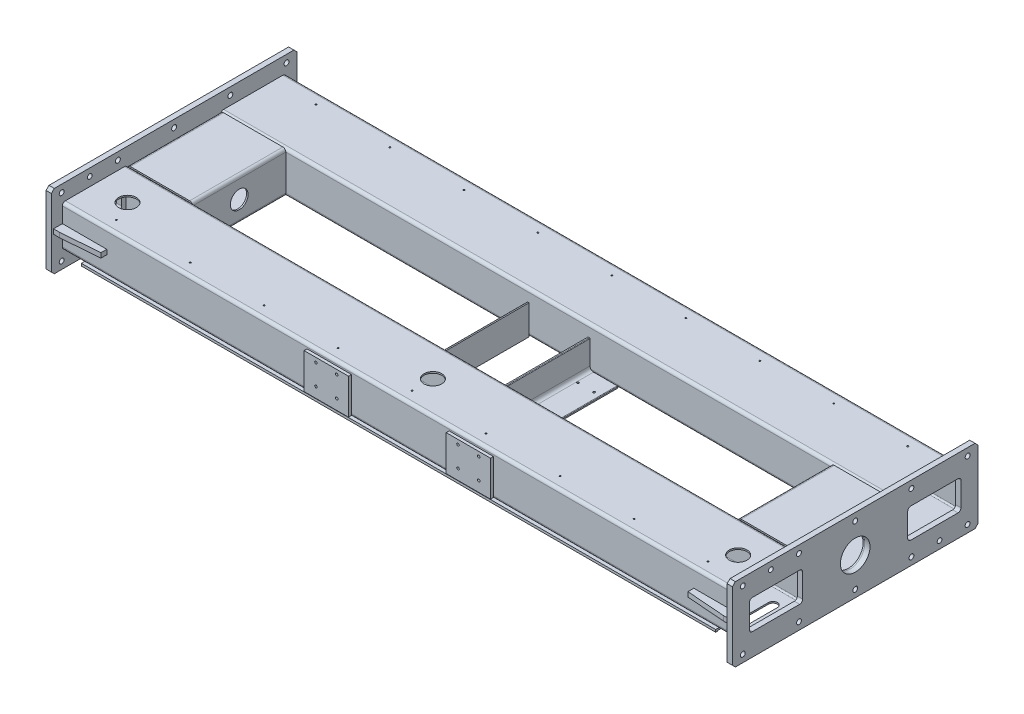
SolidWorks part; units mm, degrees
material "Q235A (2)"
ref_plane "前视基准面" through (0, 0, 0) normal (0, 0, 1) x (1, 0, 0)
ref_plane "上视基准面" through (0, 0, 0) normal (0, 1, 0) x (1, 0, 0)
ref_plane "右视基准面" through (0, 0, 0) normal (1, 0, 0) x (0, 0, -1)
sketch3d "3D草图1"
  line L0 (0, 0, 0) -> (2064, 0, 0)
  line L1 (0, 0, 0) -> (0, 0, -535)
  line L2 (2064, 0, 0) -> (2064, 0, -535)
  line L3 (0, 0, -535) -> (2064, 0, -535)
  line L4 (1032, 0, -535) -> (1032, 0, 0) construction
  line L5 (1132, 0, -535) -> (1132, 0, 0)
  line L6 (932, 0, -535) -> (932, 0, 0)
  line L15 (1132, 0, -535) -> (1132, 20, -535)
  line L16 (1132, 0, 0) -> (1132, 20, 0)
  line L17 (932, 0, 0) -> (932, 20, 0)
  line L18 (932, 0, -535) -> (932, 20, -535)
  line L19 (1132, 20, -535) -> (1132, 20, 0)
  line L20 (932, 20, 0) -> (932, 20, -535)
  line L21 (1132, 0, -535) -> (1132, -70, -535)
  line L22 (1132, 0, 0) -> (1132, -70, 0)
  line L23 (932, 0, 0) -> (932, -70, 0)
  line L24 (932, 0, -535) -> (932, -70, -535)
  line L25 (1132, -70, -535) -> (1132, -70, 0)
  line L26 (932, -70, 0) -> (932, -70, -535)
  dimension "D1" = 2064
  dimension "D2" = 535
  dimension "D3" = 200
  dimension "D4" = 100
  dimension "D5" = 20
  dimension "D6" = 70
other "矩型管 220×140×5(1)"
ref_plane "基准面1" through (0, 0, 0) normal (1, 0, 0) x (0, 1, 0)
sketch "Sketch11" plane through (0, 0, 0) normal (1, 0, 0) x (0, 1, 0)
  line L0 (-60, -105) -> (60, -105)
  line L1 (-65, -100) -> (-65, 100)
  line L2 (60, 105) -> (-60, 105)
  line L3 (65, 100) -> (65, -100)
  line L4 (-60, -110) -> (60, -110)
  line L5 (-70, -100) -> (-70, 100)
  line L6 (60, 110) -> (-60, 110)
  line L7 (70, 100) -> (70, -100)
  arc A0 (70, 100) -> (60, 110) centre (60, 100) ccw
  arc A1 (60, -110) -> (70, -100) centre (60, -100) ccw
  arc A2 (-70, -100) -> (-60, -110) centre (-60, -100) ccw
  arc A3 (-60, 110) -> (-70, 100) centre (-60, 100) ccw
  arc A4 (-60, 105) -> (-65, 100) centre (-60, 100) ccw
  arc A5 (65, 100) -> (60, 105) centre (60, 100) ccw
  arc A6 (60, -105) -> (65, -100) centre (60, -100) ccw
  arc A7 (-65, -100) -> (-60, -105) centre (-60, -100) ccw
  point P0 (0, 110)
  point P1 (70, 0)
  point P2 (0, -110)
  point P3 (-70, 0)
  point P4 (-70, 110)
  point P5 (70, 110)
  point P6 (70, -110)
  point P7 (-70, -110)
  point P8 (0, 0)
  point P33 (0, 0)
sketch "草图3" plane through (-110, 0, 0) normal (-1, 0, 0) x (0, 0, 1)
  line L0 (0, 0) -> (-535, 0) construction
  line L5 (-682.5, -125) -> (147.5, -125)
  line L6 (-682.5, -125) -> (-682.5, 125)
  line L11 (-682.5, 125) -> (147.5, 125)
  line L12 (147.5, -125) -> (147.5, 125)
  line L13 (-267.5, 125) -> (-267.5, -125) construction
  line L14 (-682.5, 0) -> (147.5, 0) construction
  point P0 (-267.5, 0)
  dimension "D1" = 250
  dimension "D2" = 830
extrude "凸台-拉伸1" add sketch "草图3" along normal blind 18 separate body
sketch "草图21" plane through (2174, 0, 0) normal (1, 0, 0) x (0, 0, -1)
  line L4 (-147.5, 125) -> (-147.5, -125)
  line L5 (-147.5, -125) -> (682.5, -125)
  line L6 (682.5, -125) -> (682.5, 125)
  line L7 (682.5, 125) -> (-147.5, 125)
  line L8 (-147.5, 125) -> (-147.5, -125)
  line L9 (-147.5, -125) -> (682.5, -125)
  line L10 (682.5, -125) -> (682.5, 125)
  line L11 (682.5, 125) -> (-147.5, 125)
  dimension "D1" = 0
extrude "凸台-拉伸4" add sketch "草图21" along normal blind 18 separate body
sketch "草图15" plane through (0, -70, 0) normal (0, -1, 0) x (1, 0, 0)
  line L0 (0, 0) -> (2064, 0) construction
  line L1 (-40, 91) -> (2104, 91) construction
  line L2 (-40, 116) -> (2104, 116)
  line L3 (-40, 116) -> (-40, 66)
  line L4 (-40, 66) -> (2104, 66)
  line L5 (2104, 116) -> (2104, 66)
  line L6 (-40, -91) -> (2104, -91) construction
  line L7 (2104, -116) -> (2104, -66)
  line L8 (-40, -66) -> (2104, -66)
  line L9 (-40, -116) -> (-40, -66)
  line L10 (-40, -116) -> (2104, -116)
  line L12 (1032, -110) -> (1032, 395.9711) construction
  line L13 (2174, -110) -> (-110, -110) construction
  line L14 (2104, -91) -> (-40, -91) construction
  line L24 (1032, -645) -> (1032, 538.6516) construction
  line L25 (2174, -645) -> (-110, -645) construction
  line L26 (-110, -425) -> (-110, -110) construction
  dimension "D1" = 70
  dimension "D2" = 50
  dimension "D3" = 182
extrude "凸台-拉伸3" add sketch "草图15" along normal blind 8 separate body
ref_plane "基准面3" through (0, 0, 80) normal (0, 0, 1) x (1, 0, 0)
ref_plane "基准面5" through (1032, 0, 0) normal (1, 0, 0) x (0, 0, -1)
sketch "草图22" plane through (0, -78, 0) normal (0, -1, 0) x (1, 0, 0)
  line L0 (-40, 116) -> (-40, 66) construction
  line L1 (-40, 66) -> (2104, 66)
  line L2 (-40, 66) -> (-40, 110)
  line L3 (-40, 110) -> (2104, 110)
  line L4 (2104, 66) -> (2104, 110)
  line L5 (-40, 66) -> (2104, 66) construction
  line L6 (2104, 66) -> (2104, 116) construction
  line L7 (2104, -66) -> (-40, -66) construction
  line L8 (-40, -66) -> (2104, -66)
  line L9 (-40, -66) -> (-40, -110)
  line L10 (-40, -110) -> (2104, -110)
  line L11 (2104, -66) -> (2104, -110)
  line L12 (2104, -116) -> (2104, -66) construction
  line L13 (0, 0) -> (2064, 0) construction
  dimension "D1" = 220
extrude "切除-拉伸1" cut sketch "草图22" against normal blind 2
hole_wizard "M8 螺纹孔1" positions "草图24" profile "草图25" tap size "M8" standard "GB"
sketch "草图24" plane through (0, -76, 0) normal (0, -1, 0) x (-1, 0, 0)
  line L0 (-2064, 0) -> (0, 0) construction
  line L2 (-2104, 91) -> (40, 91) construction
  line L3 (-2104, 110) -> (-2104, 66) construction
  line L4 (40, 66) -> (40, 110) construction
  line L6 (-2104, -91) -> (40, -91) construction
  line L7 (-1032, 91) -> (-1032, -91) construction
  point P21 (-26, 91)
  point P23 (-76, 91)
  point P25 (-176, 91)
  point P27 (-376, 91)
  point P29 (-576, 91)
  point P31 (-776, 91)
  point P34 (-876, 91)
  point P37 (-876, -91)
  point P38 (-776, -91)
  point P39 (-576, -91)
  point P40 (-376, -91)
  point P41 (-176, -91)
  point P42 (-76, -91)
  point P43 (-26, -91)
  point P44 (-2038, -91)
  point P45 (-1988, -91)
  point P46 (-1888, -91)
  point P47 (-1688, -91)
  point P48 (-1488, -91)
  point P49 (-1288, -91)
  point P50 (-1188, -91)
  point P51 (-1188, 91)
  point P52 (-1288, 91)
  point P53 (-1488, 91)
  point P54 (-1688, 91)
  point P55 (-1888, 91)
  point P56 (-1988, 91)
  point P57 (-2038, 91)
  dimension "D1" = 182
  dimension "D2" = 66
  dimension "D3" = 50
  dimension "D4" = 100
  dimension "D5" = 200
  dimension "D6" = 200
  dimension "D7" = 200
  dimension "D8" = 100
sketch "草图25" plane through (2038, -76, -91) normal (1, 0, 0) x (0, 0, -1)
  line L0 (0, 0) -> (0, 24.2929)
  line L1 (0, 24.2929) -> (3.4, 22.25)
  line L2 (3.4, 22.25) -> (3.4, 0)
  line L5 (3.4, 0) -> (0, 0)
  line L10 (0, 24.2929) -> (-3.4, 22.25) construction
  line L11 (0, -6.35) -> (0, 107.95) construction
  dimension "螺纹孔钻头直径" = 6.8
  dimension "螺纹孔钻头深度" = 22.25
  dimension "导头角度" = 118
cosmetic thread "孔螺蚊线1" parameters "D1"=11, "D2"=8
cosmetic thread "孔螺蚊线2" parameters "D1"=11, "D2"=8
cosmetic thread "孔螺蚊线3" parameters "D1"=11, "D2"=8
cosmetic thread "孔螺蚊线4" parameters "D1"=11, "D2"=8
cosmetic thread "孔螺蚊线5" parameters "D1"=11, "D2"=8
cosmetic thread "孔螺蚊线6" parameters "D1"=11, "D2"=8
cosmetic thread "孔螺蚊线7" parameters "D1"=11, "D2"=8
cosmetic thread "孔螺蚊线8" parameters "D1"=11, "D2"=8
cosmetic thread "孔螺蚊线9" parameters "D1"=11, "D2"=8
cosmetic thread "孔螺蚊线10" parameters "D1"=11, "D2"=8
cosmetic thread "孔螺蚊线11" parameters "D1"=11, "D2"=8
cosmetic thread "孔螺蚊线12" parameters "D1"=11, "D2"=8
cosmetic thread "孔螺蚊线13" parameters "D1"=11, "D2"=8
cosmetic thread "孔螺蚊线14" parameters "D1"=11, "D2"=8
cosmetic thread "孔螺蚊线15" parameters "D1"=11, "D2"=8
cosmetic thread "孔螺蚊线16" parameters "D1"=11, "D2"=8
cosmetic thread "孔螺蚊线17" parameters "D1"=11, "D2"=8
cosmetic thread "孔螺蚊线18" parameters "D1"=11, "D2"=8
cosmetic thread "孔螺蚊线19" parameters "D1"=11, "D2"=8
cosmetic thread "孔螺蚊线20" parameters "D1"=11, "D2"=8
cosmetic thread "孔螺蚊线21" parameters "D1"=11, "D2"=8
cosmetic thread "孔螺蚊线22" parameters "D1"=11, "D2"=8
cosmetic thread "孔螺蚊线23" parameters "D1"=11, "D2"=8
cosmetic thread "孔螺蚊线24" parameters "D1"=11, "D2"=8
cosmetic thread "孔螺蚊线25" parameters "D1"=11, "D2"=8
cosmetic thread "孔螺蚊线26" parameters "D1"=11, "D2"=8
cosmetic thread "孔螺蚊线27" parameters "D1"=11, "D2"=8
cosmetic thread "孔螺蚊线28" parameters "D1"=11, "D2"=8
sketch "草图27" plane through (2192, 0, 0) normal (1, 0, 0) x (0, 0, -1)
  line L0 (682.5, 0) -> (-147.5, 0) construction
  line L1 (682.5, -125) -> (682.5, 125) construction
  line L2 (-147.5, 125) -> (-147.5, -125) construction
  line L3 (535, 70) -> (535, -70) construction
  line L4 (635, 70) -> (435, 70) construction
  line L5 (435, -70) -> (635, -70) construction
  line L6 (0, 70) -> (0, -70) construction
  line L7 (100, 70) -> (-100, 70) construction
  line L8 (-100, -70) -> (100, -70) construction
  line L9 (267.5, 125) -> (267.5, -125) construction
  line L10 (455, 50) -> (615, 50)
  line L11 (445, 40) -> (445, -40)
  line L12 (455, -50) -> (615, -50)
  line L13 (625, 40) -> (625, -40)
  line L14 (535, -50) -> (535, 50) construction
  line L15 (445, 0) -> (625, 0) construction
  line L16 (682.5, 125) -> (-147.5, 125) construction
  line L17 (-147.5, -125) -> (682.5, -125) construction
  line L18 (90, 0) -> (-90, 0) construction
  line L19 (0, -50) -> (0, 50) construction
  line L20 (0, 70) -> (0, -70) construction
  line L21 (-90, 40) -> (-90, -40)
  line L22 (80, -50) -> (-80, -50)
  line L23 (90, 40) -> (90, -40)
  line L24 (80, 50) -> (-80, 50)
  arc A0 (-80, 50) -> (-90, 40) centre (-80, 40) ccw
  arc A1 (-90, -40) -> (-80, -50) centre (-80, -40) ccw
  arc A2 (80, -50) -> (90, -40) centre (80, -40) ccw
  arc A3 (80, 50) -> (90, 40) centre (80, 40) cw
  arc A4 (455, 50) -> (445, 40) centre (455, 40) ccw
  arc A5 (625, -40) -> (615, -50) centre (615, -40) cw
  arc A6 (455, -50) -> (445, -40) centre (455, -40) cw
  arc A7 (615, 50) -> (625, 40) centre (615, 40) cw
  point P18 (535, 0)
  point P36 (0, 0)
  point P39 (-90, 50)
  point P42 (-90, -50)
  point P45 (90, -50)
  point P48 (90, 50)
  point P51 (445, 50)
  point P54 (625, -50)
  point P57 (445, -50)
  point P60 (625, 50)
  dimension "D3" = 10
  dimension "D1" = 100
  dimension "D2" = 180
extrude "切除-拉伸2" cut sketch "草图27" against normal through all
sketch "草图28" plane through (-128, 0, 0) normal (-1, 0, 0) x (0, 0, 1)
  line L0 (-90, -40) -> (-90, 40) construction
  line L1 (-80, 50) -> (80, 50) construction
  line L2 (90, 40) -> (90, -40) construction
  line L3 (80, -50) -> (-80, -50) construction
  line L4 (-90, -40) -> (-90, 40)
  line L5 (-80, 50) -> (80, 50)
  line L6 (90, 40) -> (90, -40)
  line L7 (80, -50) -> (-80, -50)
  line L8 (-625, -40) -> (-625, 40) construction
  line L9 (-455, -50) -> (-615, -50) construction
  line L10 (-445, 40) -> (-445, -40) construction
  line L11 (-615, 50) -> (-455, 50) construction
  line L20 (-625, -40) -> (-625, 40)
  line L21 (-455, -50) -> (-615, -50)
  line L22 (-445, 40) -> (-445, -40)
  line L23 (-615, 50) -> (-455, 50)
  arc A0 (-80, 50) -> (-90, 40) centre (-80, 40) ccw construction
  arc A1 (90, 40) -> (80, 50) centre (80, 40) ccw construction
  arc A2 (80, -50) -> (90, -40) centre (80, -40) ccw construction
  arc A3 (-90, -40) -> (-80, -50) centre (-80, -40) ccw construction
  arc A4 (-80, 50) -> (-90, 40) centre (-80, 40) ccw
  arc A5 (90, 40) -> (80, 50) centre (80, 40) ccw
  arc A6 (80, -50) -> (90, -40) centre (80, -40) ccw
  arc A7 (-90, -40) -> (-80, -50) centre (-80, -40) ccw
  arc A8 (-615, 50) -> (-625, 40) centre (-615, 40) ccw construction
  arc A9 (-625, -40) -> (-615, -50) centre (-615, -40) ccw construction
  arc A10 (-455, -50) -> (-445, -40) centre (-455, -40) ccw construction
  arc A11 (-445, 40) -> (-455, 50) centre (-455, 40) ccw construction
  arc A12 (-615, 50) -> (-625, 40) centre (-615, 40) ccw
  arc A13 (-625, -40) -> (-615, -50) centre (-615, -40) ccw
  arc A14 (-455, -50) -> (-445, -40) centre (-455, -40) ccw
  arc A15 (-445, 40) -> (-455, 50) centre (-455, 40) ccw
extrude "切除-拉伸3" cut sketch "草图28" against normal blind 25
sketch "草图29" plane through (0, -70, 0) normal (0, -1, 0) x (1, 0, 0)
  line L0 (0, 0) -> (2064, 0) construction
  line L1 (1107, 0) -> (957, 0) construction
  line L2 (1107, -45) -> (957, -45)
  line L3 (1107, 45) -> (957, 45)
  arc A0 (1107, -45) -> (1107, 45) centre (1107, 0) ccw
  arc A1 (957, 45) -> (957, -45) centre (957, 0) ccw
  point P6 (1032, 0)
  dimension "D1" = 90
  dimension "D2" = 150
extrude "切除-拉伸4" cut sketch "草图29" against normal blind 6
sketch "草图30" plane through (0, 0, 0) normal (0, 1, 0) x (1, 0, 0)
  line L8 (-128, 267.5) -> (2192, 267.5) construction
  line L9 (-128, -147.5) -> (-128, 682.5) construction
  line L10 (2192, 682.5) -> (2192, -147.5) construction
  line L17 (1032, 535) -> (1032, -585.4821) construction
  line L18 (0, 535) -> (2064, 535) construction
  line L19 (1032, -137.5) -> (1032, 137.5) construction
hole_wizard "Ø16.5 (16.5) 直径孔1" positions "草图32" profile "草图33" hole size "Ø16.5" standard "GB"
sketch "草图32" plane through (2192, 0, 0) normal (1, 0, 0) x (0, 0, -1)
  line L1 (647.5, -100) -> (-112.5, -100) construction
  line L2 (647.5, -100) -> (647.5, 100) construction
  line L3 (647.5, 100) -> (-112.5, 100) construction
  line L4 (-112.5, -100) -> (-112.5, 100) construction
  line L5 (267.5, 100) -> (267.5, -100) construction
  line L6 (647.5, 0) -> (-112.5, 0) construction
  line L8 (267.5, 125) -> (267.5, -125) construction
  line L9 (682.5, 125) -> (-147.5, 125) construction
  line L10 (-147.5, -125) -> (682.5, -125) construction
  line L11 (77.5, 100) -> (77.5, -100) construction
  line L13 (457.5, 100) -> (457.5, -100) construction
  point P2 (-112.5, 100)
  point P279 (647.5, -100)
  point P280 (647.5, 100)
  point P281 (-112.5, -100)
  point P283 (267.5, -100)
  point P285 (267.5, 100)
  point P308 (457.5, 100)
  point P310 (77.5, 100)
  point P314 (77.5, -100)
  point P317 (457.5, -100)
  point P319 (350.269, 181.4428)
  point P321 (350.269, 181.4428)
  dimension "D1" = 760
  dimension "D2" = 200
  dimension "D3" = 380
sketch "草图33" plane through (2192, 100, 112.5) normal (0, 1, 0) x (0, 0, -1)
  line L0 (0, 0) -> (0, 2320)
  line L1 (0, 2320) -> (8.25, 2320)
  line L2 (8.25, 2320) -> (8.25, 0)
  line L5 (8.25, 0) -> (0, 0)
  line L11 (0, -6.35) -> (0, 107.95) construction
  dimension "通孔孔直径" = 16.5
  dimension "通孔孔深度" = 2320
hole_wizard "大小mm 暗销孔1" positions "草图34" profile "草图35" hole size "Ø16.0" standard "GB" end condition through all
sketch "草图34" plane through (2192, 0, 0) normal (1, 0, 0) x (0, 0, -1)
  line L0 (-112.5, 100) -> (77.5, 100) construction
  line L2 (457.5, -100) -> (647.5, -100) construction
  point P13 (-17.5, 100)
  point P15 (552.5, -100)
sketch "草图35" plane through (2192, -100, -552.5) normal (0, 1, 0) x (0, 0, -1)
  line L0 (0, 0) -> (0, 2320)
  line L1 (0, 2320) -> (8, 2320)
  line L2 (8, 2320) -> (8, 0)
  line L5 (8, 0) -> (0, 0)
  line L11 (0, -6.35) -> (0, 107.95) construction
  dimension "通孔孔直径" = 16
  dimension "通孔孔深度" = 2320
chamfer "倒角1" distance 10 angle 45 4 edges at (2183, 125, -682.5) (2183, -125, -682.5) (2183, 125, 147.5) (2183, -125, 147.5)
chamfer "倒角2" distance 10 angle 45 4 edges at (-119, -125, 147.5) (-119, 125, 147.5) (-119, 125, -682.5) (-119, -125, -682.5)
ref_plane "基准面6" through (0, 0, -535) normal (0, 0, -1) x (-1, 0, 0)
other "等边角钢 10×6(4)"
ref_plane "基准面7" through (1132, -70, -535) normal (0, 0, 1) x (0, 1, 0)
sketch "Sketch1" plane through (1132, -70, -535) normal (0, 0, 1) x (0, 1, 0)
  line L0 (100, 0) -> (0, 0)
  line L1 (0, 0) -> (0, -100)
  line L2 (98, -6) -> (18, -6)
  line L3 (6, -18) -> (6, -98)
  line L4 (100, 0) -> (100, -4)
  line L5 (0, -100) -> (4, -100)
  arc A0 (100, -4) -> (98, -6) centre (98, -4) cw
  arc A1 (4, -100) -> (6, -98) centre (4, -98) ccw
  arc A2 (18, -6) -> (6, -18) centre (18, -18) ccw
  point P2 (50, 0)
  point P13 (0, -50)
  point P15 (0, 0)
  dimension "r1" = 2
  dimension "r" = 12
  dimension "b" = 100
  dimension "d" = 6
other "等边角钢 10×6(1)"
ref_plane "基准面8" through (932, -70, 0) normal (0, 0, 1) x (-1, 0, 0)
sketch "Sketch15" plane through (932, -70, 0) normal (0, 0, 1) x (-1, 0, 0)
  line L0 (100, 0) -> (0, 0)
  line L1 (0, 0) -> (0, -100)
  line L2 (98, -6) -> (18, -6)
  line L3 (6, -18) -> (6, -98)
  line L4 (100, 0) -> (100, -4)
  line L5 (0, -100) -> (4, -100)
  arc A0 (100, -4) -> (98, -6) centre (98, -4) cw
  arc A1 (4, -100) -> (6, -98) centre (4, -98) ccw
  arc A2 (18, -6) -> (6, -18) centre (18, -18) ccw
  point P2 (50, 0)
  point P13 (0, -50)
  point P15 (0, 0)
  dimension "r1" = 2
  dimension "r" = 12
  dimension "b" = 100
  dimension "d" = 6
other "剪裁/延伸1"
sketch "草图41" plane through (0, 0, 0) normal (0, 1, 0) x (1, 0, 0)
  line L0 (2174, -110) -> (-110, -110) construction
  line L1 (40, -110) -> (-110, -110)
  line L2 (-110, -110) -> (-110, -140)
  line L3 (-90, 675) -> (-110, 675)
  line L4 (40, -110) -> (40, -130)
  line L5 (40, -130) -> (-90, -140)
  line L6 (-90, -140) -> (-110, -140)
  line L7 (-110, -137.5) -> (-110, -147.5) construction
  line L8 (2174, -100) -> (-110, -100) construction
  line L9 (1032, 535) -> (1032, -585.4821) construction
  line L10 (-128, 267.5) -> (2192, 267.5) construction
  line L26 (40, 665) -> (-90, 675)
  line L27 (40, 645) -> (40, 665)
  line L28 (-110, 645) -> (-110, 675)
  line L29 (40, 645) -> (-110, 645)
  line L30 (2024, 645) -> (2174, 645)
  line L31 (2174, 645) -> (2174, 675)
  line L32 (2024, 645) -> (2024, 665)
  line L33 (2024, 665) -> (2154, 675)
  line L34 (2154, -140) -> (2174, -140)
  line L35 (2024, -130) -> (2154, -140)
  line L36 (2024, -110) -> (2024, -130)
  line L37 (2154, 675) -> (2174, 675)
  line L39 (2024, -110) -> (2174, -110)
  line L40 (2174, -140) -> (2174, -110)
  dimension "D1" = 20
  dimension "D2" = 150
  dimension "D3" = 20
  dimension "D4" = 40
extrude "凸台-拉伸7" add sketch "草图41" along normal mid plane 16 separate body
sketch "草图42" plane through (0, 70, 0) normal (0, 1, 0) x (1, 0, 0)
  line L0 (1032, 535) -> (1032, -585.4821) construction
  line L1 (32, -70) -> (2032, -70) construction
  line L2 (2174, -110) -> (2024, -110) construction
  point P6 (782, -70)
  point P9 (1032, -70)
  point P10 (532, -70)
  point P11 (1782, -70)
  point P13 (32, -70)
  point P14 (1532, -70)
  point P15 (282, -70)
  point P16 (1282, -70)
  dimension "D1" = 40
  dimension "D2" = 250
  dimension "D3" = 250
  dimension "D4" = 250
  dimension "D5" = 250
hole_wizard "M6 螺纹孔2" positions "草图47" profile "草图48" tap size "M6" standard "GB"
sketch "草图47" plane through (0, 70, 0) normal (0, 1, 0) x (1, 0, 0)
  line L1 (1032, 535) -> (1032, -70) construction
  line L2 (-128, 267.5) -> (2192, 267.5) construction
  line L3 (32, 605) -> (2032, 605) construction
  point P5 (1032, -70)
  point P13 (32, -70)
  point P16 (282, -70)
  point P19 (532, -70)
  point P22 (782, -70)
  point P27 (1282, -70)
  point P30 (1532, -70)
  point P33 (1782, -70)
  point P36 (2032, -70)
  point P40 (2032, 605)
  point P41 (1782, 605)
  point P42 (1532, 605)
  point P43 (1282, 605)
  point P44 (782, 605)
  point P45 (532, 605)
  point P46 (282, 605)
  point P47 (32, 605)
  point P48 (1032, 605)
sketch "草图48" plane through (1032, 70, -605) normal (1, 0, 0) x (0, 0, 1)
  line L0 (0, 0) -> (0, 18.5022)
  line L1 (0, 18.5022) -> (2.5, 17)
  line L2 (2.5, 17) -> (2.5, 0)
  line L5 (2.5, 0) -> (0, 0)
  line L10 (0, 18.5022) -> (-2.5, 17) construction
  line L11 (0, -6.35) -> (0, 107.95) construction
  dimension "螺纹孔钻头直径" = 5
  dimension "螺纹孔钻头深度" = 17
  dimension "导头角度" = 118
cosmetic thread "孔螺蚊线45" parameters "D1"=5, "D2"=6
cosmetic thread "孔螺蚊线46" parameters "D1"=5, "D2"=6
cosmetic thread "孔螺蚊线47" parameters "D1"=5, "D2"=6
cosmetic thread "孔螺蚊线48" parameters "D1"=5, "D2"=6
cosmetic thread "孔螺蚊线49" parameters "D1"=5, "D2"=6
cosmetic thread "孔螺蚊线50" parameters "D1"=5, "D2"=6
cosmetic thread "孔螺蚊线51" parameters "D1"=5, "D2"=6
cosmetic thread "孔螺蚊线52" parameters "D1"=5, "D2"=6
cosmetic thread "孔螺蚊线53" parameters "D1"=5, "D2"=6
cosmetic thread "孔螺蚊线54" parameters "D1"=5, "D2"=6
cosmetic thread "孔螺蚊线55" parameters "D1"=5, "D2"=6
cosmetic thread "孔螺蚊线56" parameters "D1"=5, "D2"=6
cosmetic thread "孔螺蚊线57" parameters "D1"=5, "D2"=6
cosmetic thread "孔螺蚊线58" parameters "D1"=5, "D2"=6
cosmetic thread "孔螺蚊线59" parameters "D1"=5, "D2"=6
cosmetic thread "孔螺蚊线60" parameters "D1"=5, "D2"=6
cosmetic thread "孔螺蚊线61" parameters "D1"=5, "D2"=6
cosmetic thread "孔螺蚊线62" parameters "D1"=5, "D2"=6
hole_wizard "M8 螺纹孔3" positions "草图49" profile "草图50" tap size "M8" standard "GB"
sketch "草图49" plane through (0, -70, 0) normal (0, -1, 0) x (-1, 0, 0)
  line L2 (-1182, 167.5) -> (-882, 167.5) construction
  line L3 (-1182, 167.5) -> (-1182, 367.5) construction
  line L4 (-1182, 367.5) -> (-882, 367.5) construction
  line L5 (-882, 167.5) -> (-882, 367.5) construction
  line L6 (-1032, 367.5) -> (-1032, 167.5) construction
  line L7 (-1182, 267.5) -> (-882, 267.5) construction
  line L8 (-1182, 367.5) -> (-1209.5, 367.5) construction
  line L9 (-1154.5, 167.5) -> (-1209.5, 167.5) construction
  line L10 (-882, 367.5) -> (-854.5, 367.5) construction
  line L11 (-882, 167.5) -> (-854.5, 167.5) construction
  line L12 (128, 267.5) -> (-2192, 267.5) construction
  line L13 (-854.5, 367.5) -> (-854.5, 167.5) construction
  line L14 (-909.5, 367.5) -> (-909.5, 167.5) construction
  line L16 (-1154.5, 367.5) -> (-1154.5, 167.5) construction
  line L17 (-1209.5, 367.5) -> (-1209.5, 167.5) construction
  point P233 (-1209.5, 367.5)
  point P236 (-1209.5, 167.5)
  point P239 (-854.5, 367.5)
  point P242 (-854.5, 167.5)
  point P252 (-909.5, 367.5)
  point P254 (-1154.5, 367.5)
  point P256 (-1154.5, 167.5)
  point P258 (-909.5, 167.5)
  dimension "D1" = 300
  dimension "D2" = 200
  dimension "D3" = 27.5
  dimension "D4" = 55
sketch "草图50" plane through (909.5, -70, -167.5) normal (1, 0, 0) x (0, 0, -1)
  line L0 (0, 0) -> (0, 24.2929)
  line L1 (0, 24.2929) -> (3.4, 22.25)
  line L2 (3.4, 22.25) -> (3.4, 0)
  line L5 (3.4, 0) -> (0, 0)
  line L10 (0, 24.2929) -> (-3.4, 22.25) construction
  line L11 (0, -6.35) -> (0, 107.95) construction
  dimension "螺纹孔钻头直径" = 6.8
  dimension "螺纹孔钻头深度" = 22.25
  dimension "导头角度" = 118
cosmetic thread "孔螺蚊线37" parameters "D1"=6, "D2"=8
cosmetic thread "孔螺蚊线38" parameters "D1"=6, "D2"=8
cosmetic thread "孔螺蚊线39" parameters "D1"=6, "D2"=8
cosmetic thread "孔螺蚊线40" parameters "D1"=6, "D2"=8
cosmetic thread "孔螺蚊线41" parameters "D1"=6, "D2"=8
cosmetic thread "孔螺蚊线42" parameters "D1"=6, "D2"=8
cosmetic thread "孔螺蚊线43" parameters "D1"=6, "D2"=8
cosmetic thread "孔螺蚊线44" parameters "D1"=6, "D2"=8
sketch "草图52" plane through (0, 70, 0) normal (0, 1, 0) x (1, 0, 0)
  circle A0 centre (2064, 0) radius 30
  circle A1 centre (0, 0) radius 30
  circle A2 centre (1032, 0) radius 30
  dimension "D1" = 60
extrude "切除-拉伸6" cut sketch "草图52" against normal blind 10
sketch "草图53" plane through (2192, 0, 0) normal (1, 0, 0) x (0, 0, -1)
  line L0 (0, 0) -> (535, 0) construction
  circle A0 centre (267.5, 0) radius 50
  dimension "D1" = 100
extrude "切除-拉伸7" cut sketch "草图53" against normal blind 50
sketch "草图54" plane through (-128, 0, 0) normal (-1, 0, 0) x (0, 0, 1)
  line L0 (0, 0) -> (-535, 0) construction
  circle A0 centre (-267.5, 0) radius 50
  dimension "D1" = 100
extrude "切除-拉伸8" cut sketch "草图54" against normal blind 50
sketch "草图55" plane through (0, 0, 110) normal (0, 0, 1) x (1, 0, 0)
  line L0 (1032, -78) -> (1032, 70) construction
  line L1 (2104, -78) -> (-40, -78) construction
  line L3 (867, -65) -> (717, -65)
  line L4 (867, -65) -> (867, 55)
  line L5 (867, 55) -> (717, 55)
  line L6 (717, -65) -> (717, 55)
  line L7 (792, 55) -> (792, -65) construction
  line L8 (867, -5) -> (717, -5) construction
  line L9 (1197, -5) -> (1347, -5) construction
  line L10 (1272, 55) -> (1272, -65) construction
  line L11 (1347, -65) -> (1347, 55)
  line L12 (1197, 55) -> (1347, 55)
  line L13 (1197, -65) -> (1197, 55)
  line L14 (1197, -65) -> (1347, -65)
  point P5 (792, -5)
  point P19 (1272, -5)
  dimension "D1" = 150
  dimension "D2" = 15
  dimension "500" = 480
  dimension "D4" = 120
extrude "凸台-拉伸8" add sketch "草图55" along normal blind 10 separate body
hole_wizard "M10 螺纹孔1" positions "草图56" profile "草图57" tap size "M10" standard "GB"
sketch "草图56" plane through (0, 0, 120) normal (0, 0, 1) x (1, 0, 0)
  line L0 (1272, 55) -> (1272, -65) construction
  line L1 (1347, 55) -> (1197, 55) construction
  line L2 (1197, -65) -> (1347, -65) construction
  line L3 (792, 55) -> (792, -65) construction
  line L4 (867, 55) -> (717, 55) construction
  line L5 (717, -65) -> (867, -65) construction
  line L7 (757, -30) -> (827, -30) construction
  line L8 (757, -30) -> (757, 40) construction
  line L9 (757, 40) -> (827, 40) construction
  line L10 (827, -30) -> (827, 40) construction
  line L11 (792, 40) -> (792, -30) construction
  line L12 (757, 5) -> (827, 5) construction
  line L15 (1032, 70) -> (1032, -78) construction
  line L16 (2104, -78) -> (-40, -78) construction
  line L17 (1357, -5) -> (1231.4436, -5) construction
  line L18 (1307, 5) -> (1237, 5) construction
  line L19 (1272, 40) -> (1272, -30) construction
  line L20 (1237, -30) -> (1237, 40) construction
  line L21 (1307, 40) -> (1237, 40) construction
  line L22 (1307, -30) -> (1307, 40) construction
  line L23 (1307, -30) -> (1237, -30) construction
  line L24 (1272, 55) -> (1272, -65) construction
  point P16 (827, 40)
  point P173 (757, -30)
  point P174 (757, 40)
  point P175 (827, -30)
  point P210 (1237, -30)
  point P211 (1237, 40)
  point P212 (1307, 40)
  point P213 (1307, -30)
  dimension "D1" = 70
  dimension "D2" = 70
  dimension "D3" = 15
sketch "草图57" plane through (1307, -30, 120) normal (1, 0, 0) x (0, -1, 0)
  line L0 (0, 0) -> (0, 30.0537)
  line L1 (0, 30.0537) -> (4.25, 27.5)
  line L2 (4.25, 27.5) -> (4.25, 0)
  line L5 (4.25, 0) -> (0, 0)
  line L10 (0, 30.0537) -> (-4.25, 27.5) construction
  line L11 (0, -6.35) -> (0, 107.95) construction
  dimension "螺纹孔钻头直径" = 8.5
  dimension "螺纹孔钻头深度" = 27.5
  dimension "导头角度" = 118
cosmetic thread "孔螺蚊线29" parameters "D1"=15, "D2"=10
cosmetic thread "孔螺蚊线30" parameters "D1"=15, "D2"=10
cosmetic thread "孔螺蚊线31" parameters "D1"=15, "D2"=10
cosmetic thread "孔螺蚊线32" parameters "D1"=15, "D2"=10
cosmetic thread "孔螺蚊线33" parameters "D1"=15, "D2"=10
cosmetic thread "孔螺蚊线34" parameters "D1"=15, "D2"=10
cosmetic thread "孔螺蚊线35" parameters "D1"=15, "D2"=10
cosmetic thread "孔螺蚊线36" parameters "D1"=15, "D2"=10
sketch "草图58" plane through (110, 0, 0) normal (1, 0, 0) x (0, 0, -1)
  circle A0 centre (267.5, 0) radius 30
extrude "切除-拉伸9" cut sketch "草图58" against normal blind 10
sketch "草图59" plane through (1954, 0, 0) normal (-1, 0, 0) x (0, 0, 1)
  circle A0 centre (-267.5, 0) radius 30 construction
  circle A1 centre (-267.5, 0) radius 30
extrude "切除-拉伸10" cut sketch "草图59" against normal blind 10
sketch "草图60" plane through (0, -70, 0) normal (0, -1, 0) x (1, 0, 0)
  line L0 (0, 0) -> (2134, 0) construction
  line L1 (2134, -47.5) -> (2134, 47.5) construction
  line L2 (2119, -47.5) -> (2119, 47.5)
  line L3 (2149, -47.5) -> (2149, 47.5)
  line L4 (2174, 100) -> (2174, -100) construction
  line L5 (1032, 585.4821) -> (1032, -772.0317) construction
  line L6 (-70, -47.5) -> (-70, 47.5) construction
  line L7 (-55, -47.5) -> (-55, 47.5)
  line L8 (-85, -47.5) -> (-85, 47.5)
  arc A1 (2119, -47.5) -> (2149, -47.5) centre (2134, -47.5) ccw
  arc A2 (2149, 47.5) -> (2119, 47.5) centre (2134, 47.5) ccw
  arc A3 (-55, -47.5) -> (-85, -47.5) centre (-70, -47.5) cw
  arc A4 (-85, 47.5) -> (-55, 47.5) centre (-70, 47.5) cw
  point P4 (2134, 0)
  point P17 (-70, 0)
  dimension "D1" = 30
  dimension "D2" = 95
  dimension "D3" = 40
extrude "切除-拉伸11" cut sketch "草图60" against normal blind 5
equation "\"D1@Sketch11\" = \"Thickness@Sketch11\" * 2"
